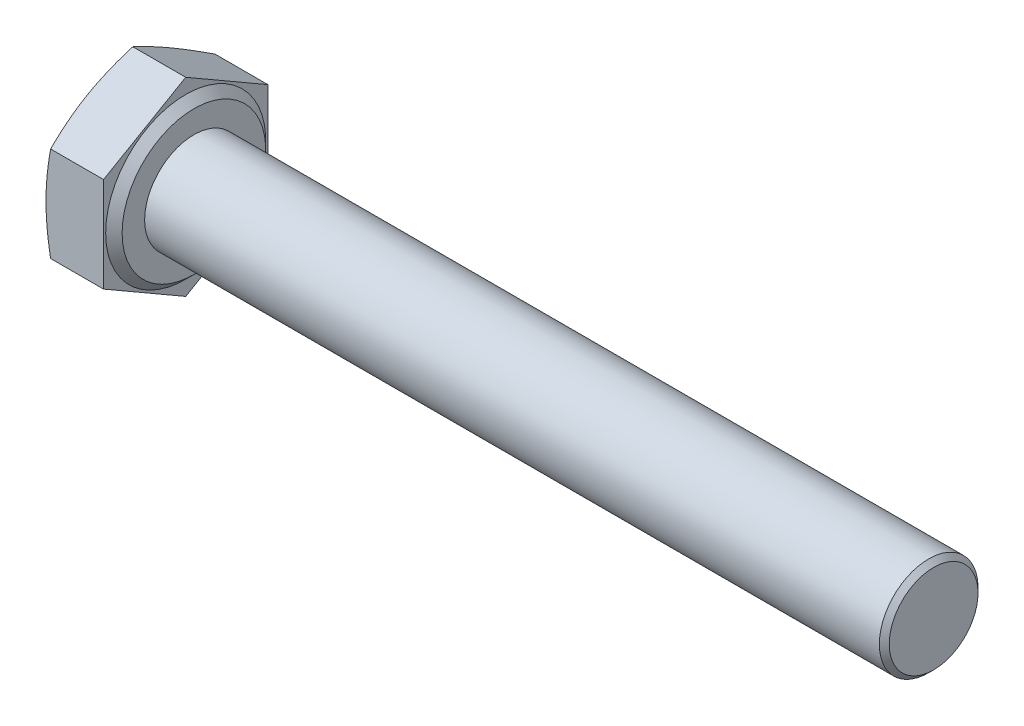
from build123d import *

# Parameters (mm, degrees)
BASEHEAD_DEPTH = 4
SKETCH5_R      = 3
BASEBODY_DEPTH = 45
CHAMFER1_SIZE  = 0.3


with BuildPart() as part:
    # Sketch2 → BaseHead (new body)
    with BuildSketch(Plane(origin=(0, 0, 0), x_dir=(0, 0, -1), z_dir=(1, 0, 0))):
        Polygon((0, -5.773502692), (5, -2.886751346), (5, 2.886751346), (0, 5.773502692), (-5, 2.886751346), (-5, -2.886751346), align=None)
    extrude(amount=BASEHEAD_DEPTH)

    # Sketch3 → BearingFace (revolve, cut)
    with BuildSketch(Plane.XY, mode=Mode.PRIVATE) as bearingface_sk:
        Polygon((4, 5.773502692), (4, 4.37), (3.5, 4.87), (3.5, 5.773502692), align=None)
    revolve(bearingface_sk.sketch.rotate(Axis((-0.957090588, 0, 0), (1, 0, 0)), 90), axis=Axis((-0.957090588, 0, 0), (1, 0, 0)), mode=Mode.SUBTRACT)

    # Sketch4 → HeadChamfer (revolve, cut)
    with BuildSketch(Plane.XY):
        Polygon((0, 5.773502692), (0.281531956, 5.773502692), (0, 5), align=None)
    revolve(axis=Axis((-0.493528746, 0, 0), (1, 0, 0)), mode=Mode.SUBTRACT)

    # Sketch5 → BaseBody (add)
    with BuildSketch(Plane(origin=(4, 0, 0), x_dir=(0, 0, -1), z_dir=(1, 0, 0))):
        with Locations(Location((0, 0, 0), (0, 0, 180))):
            Circle(SKETCH5_R)
    extrude(amount=BASEBODY_DEPTH)

    # Chamfer1
    chamfer1_edges = [part.edges().sort_by_distance(p)[0] for p in [
        (49, 0, -3),
    ]]
    chamfer(chamfer1_edges, length=CHAMFER1_SIZE)


solid = part.part
